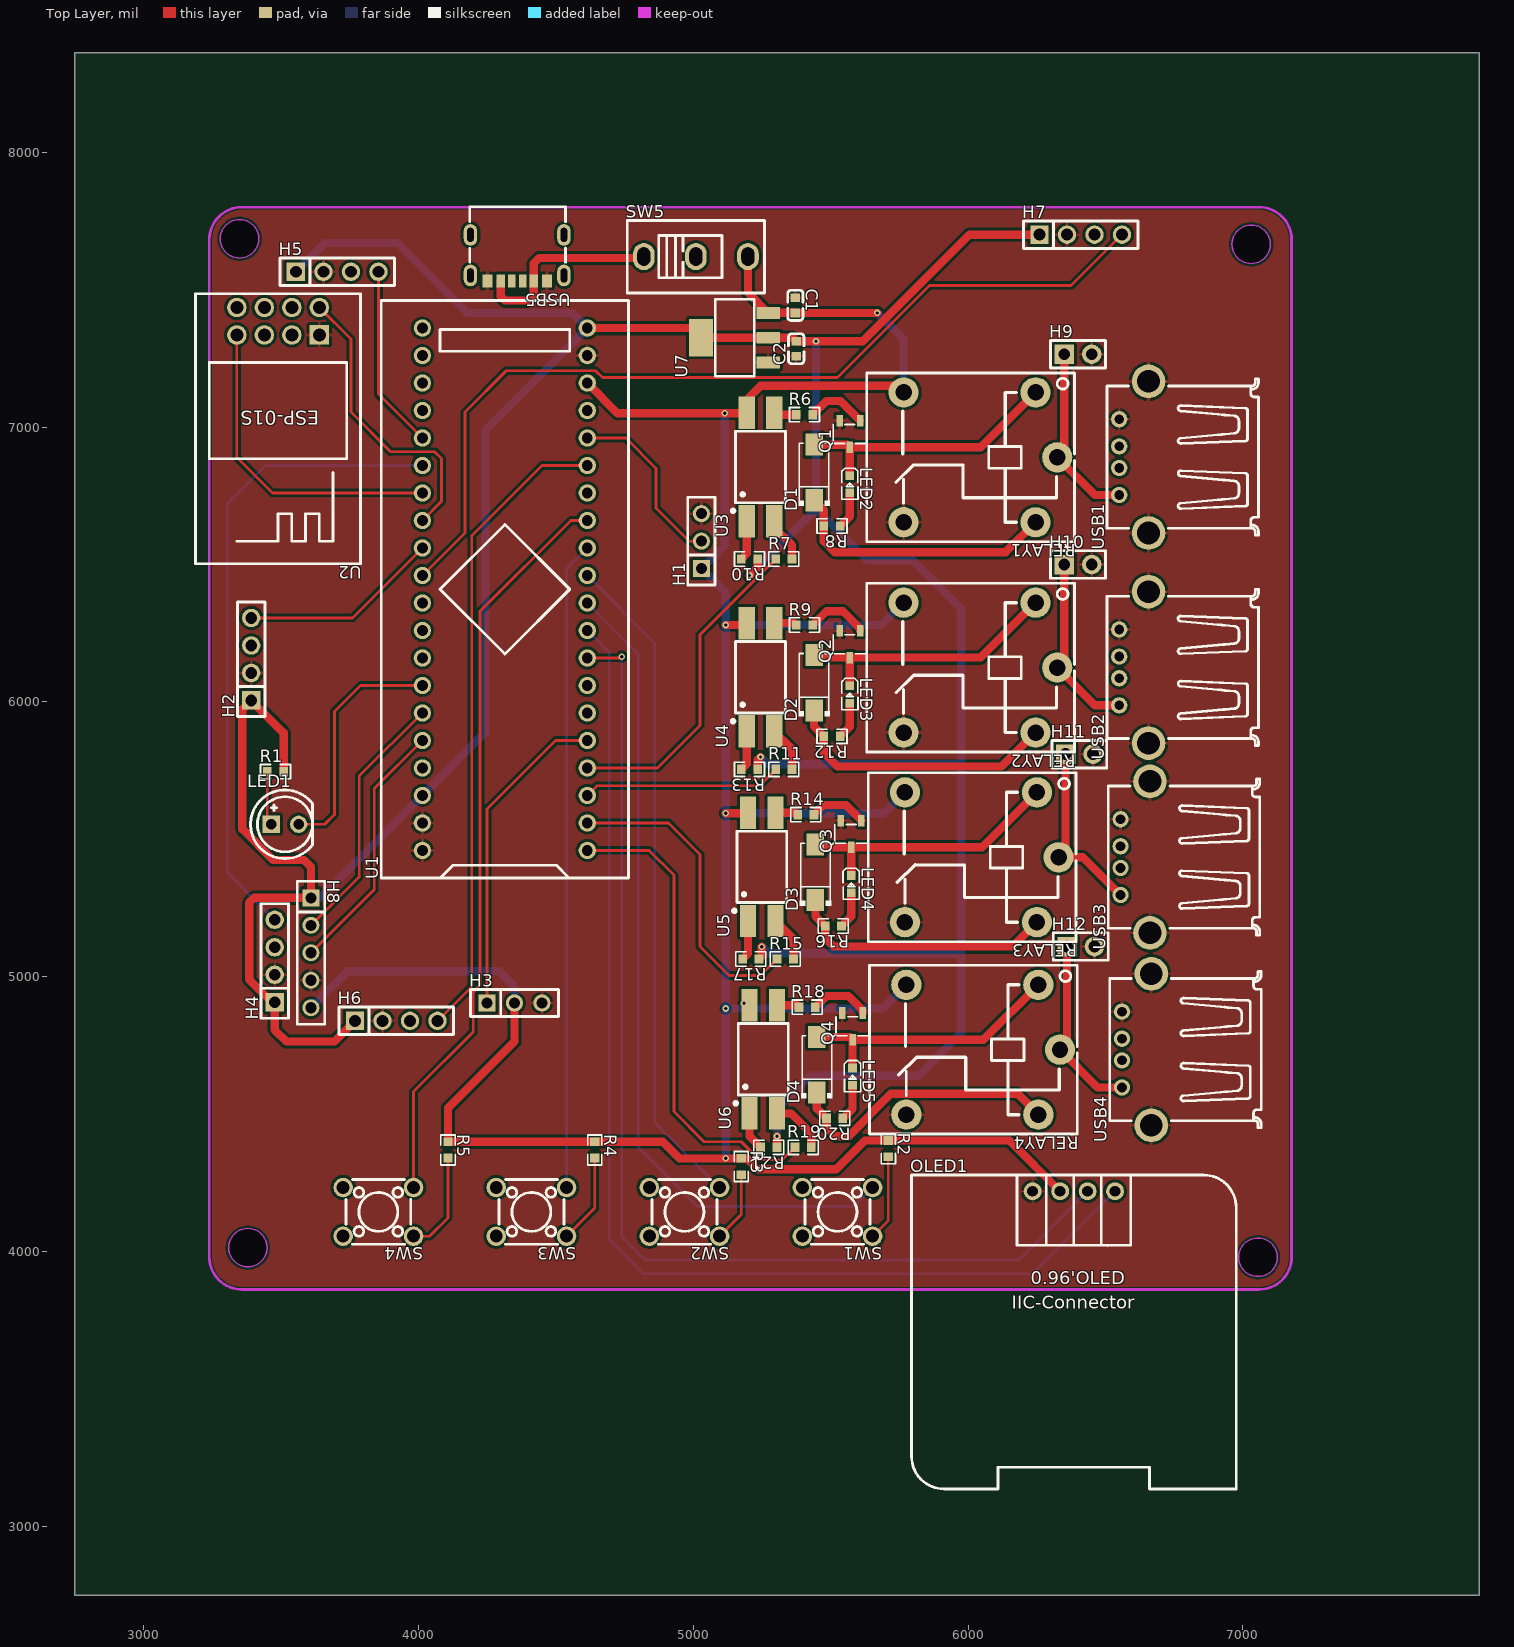
[diagram p0: Top Layer view]
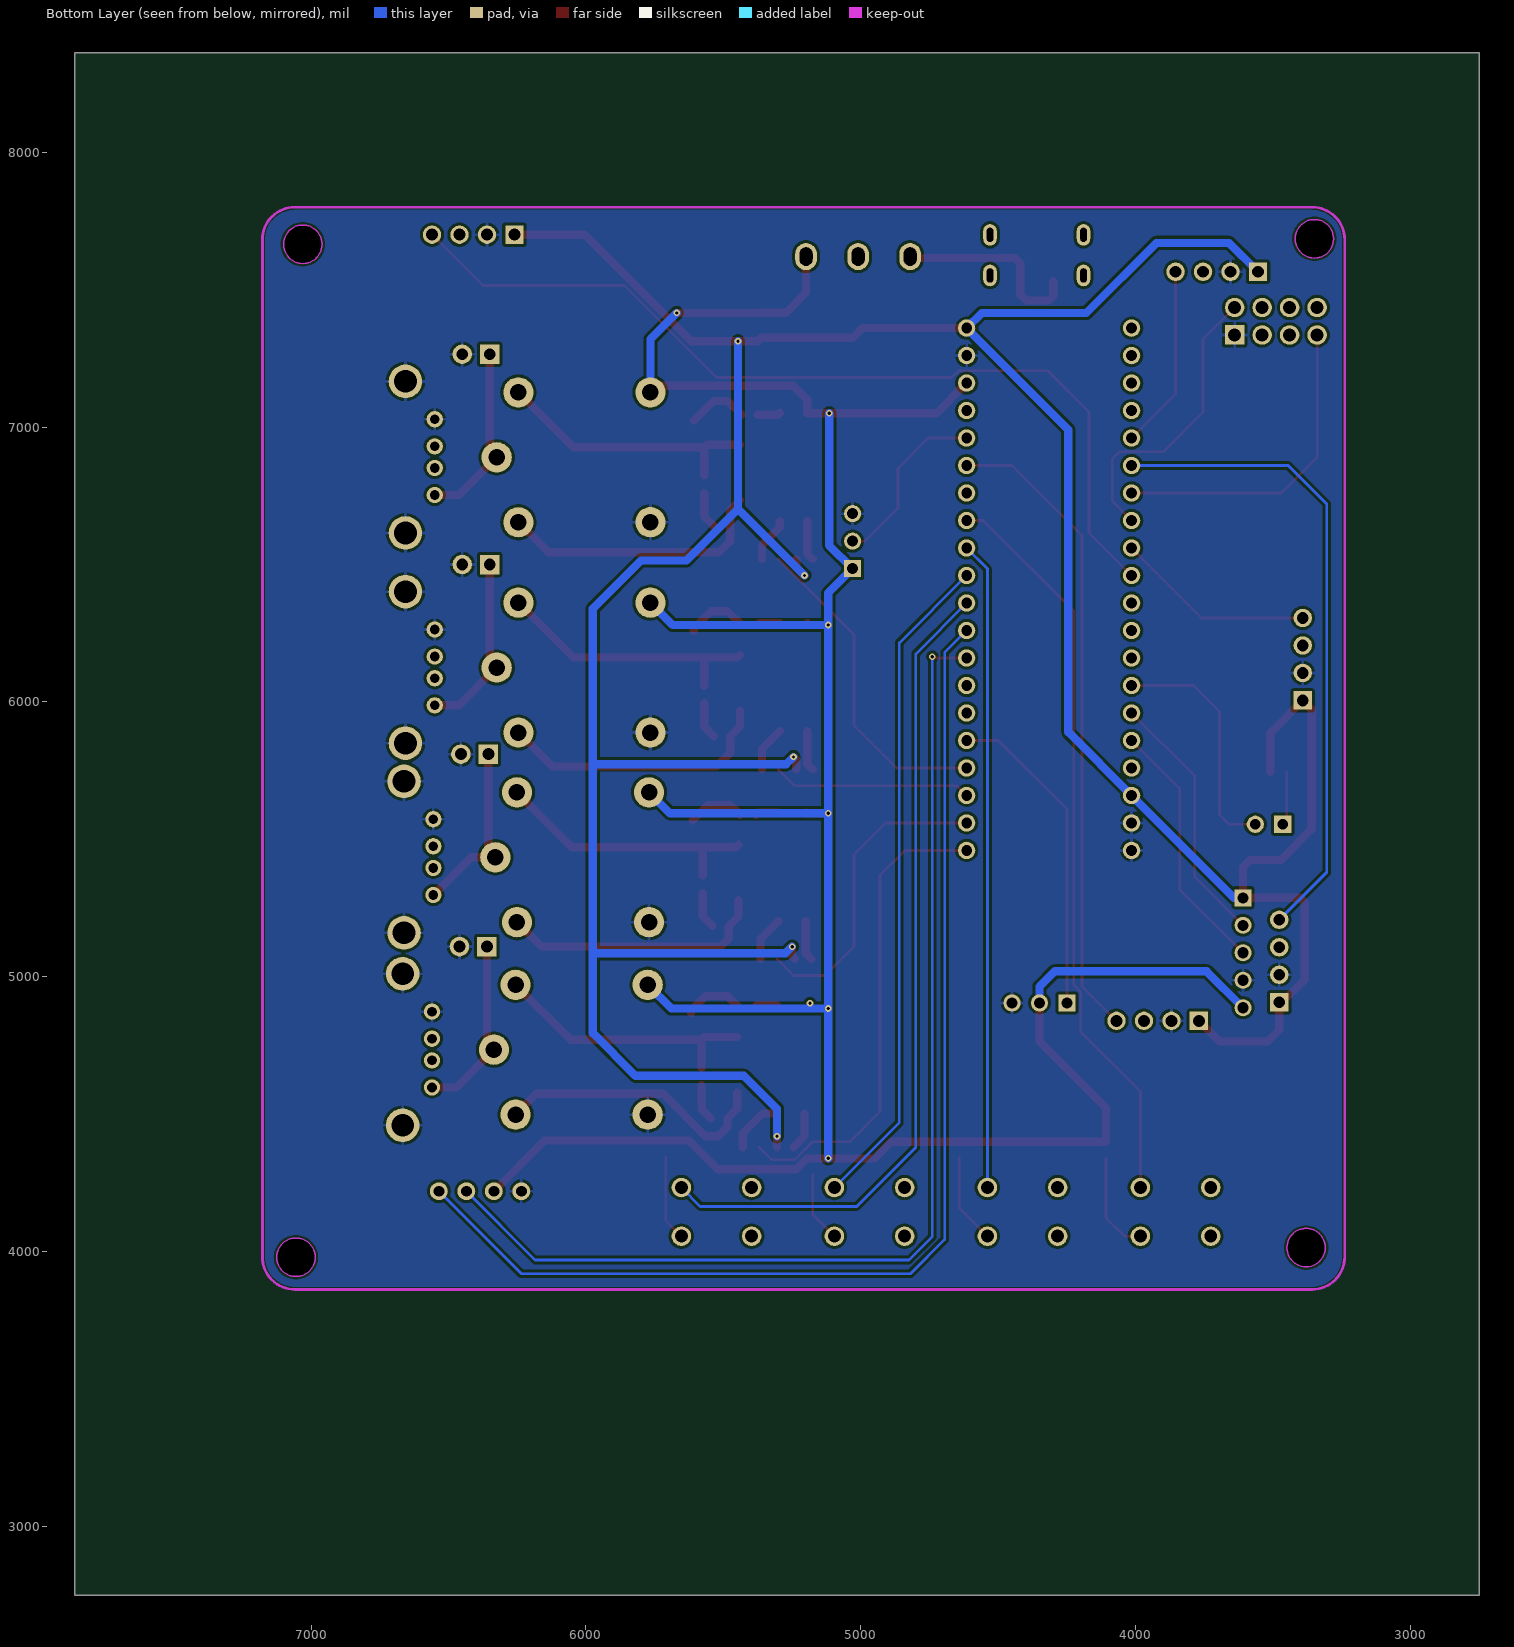
[diagram p1: Bottom Layer view, seen from below]
# Altium PCB MISC51241.pcbdoc
Units mil, origin at the board's own origin, x right, y up, seen from the top; angles counter-clockwise.
Board outline 5110 x 5612.11 mil, 2 copper layers (Top Layer, Bottom Layer), stack 62.206 mil thick; 70 components, 76 nets, 260 pads, 13 vias.

## Layer stack, top to bottom
Top Solder Mask Layer: solder mask 0.394, Dk 3.3
Top Layer: signal copper 1.379
Dielectric1: surface 59.449, FR4, Dk 4.5
Bottom Layer: signal copper 1.378
Bottom Solder Mask Layer: solder mask 0.394, Dk 3.3

## Board outline
7860,2750 2750,2750 2750,8362.11 7860,8362.11
cut-out: 3420,7685 cw(c3350,7685) 3280,7685 cw(c3350,7685)
cut-out: 3450,4015 cw(c3380,4015) 3310,4015 cw(c3380,4015)
cut-out: 7125,3980 cw(c7055,3980) 6985,3980 cw(c7055,3980)
cut-out: 7100,7665 cw(c7030,7665) 6960,7665 cw(c7030,7665)

## Design rules (kind name [scope] priority, off if disabled: settings)
BoardOutlineClearance copperThickness2oz_1 [All] p2 off: genericclearance=7.99 ignorepadtopadclearanceinfootprint=FALSE except(0: Arc-SplitContinuation Track-SplitContinuation SMDPad-SplitContinuation THPad-SplitContinuation Via-SplitContinuation Fill-SplitContinuation Region-SplitContinuation Poly-SplitContinuation Text-SplitContinuation Hole-SplitContinuation; 5.98: Arc-CutoutEdge Track-CutoutEdge SMDPad-CutoutEdge THPad-CutoutEdge Via-CutoutEdge Text-CutoutEdge; 6.9: Hole-OutlineEdge Hole-CutoutEdge; 10: Poly-OutlineEdge Poly-CutoutEdge; 11.81: Arc-OutlineEdge Track-OutlineEdge SMDPad-OutlineEdge THPad-OutlineEdge Via-OutlineEdge Fill-OutlineEdge Region-OutlineEdge Text-OutlineEdge Fill-CutoutEdge Region-CutoutEdge)
BoardOutlineClearance Plane_innerPlane_1 [All] p4 off: genericclearance=4.02 ignorepadtopadclearanceinfootprint=FALSE except(0: Arc-SplitContinuation Track-SplitContinuation SMDPad-SplitContinuation THPad-SplitContinuation Via-SplitContinuation Fill-SplitContinuation Region-SplitContinuation Poly-SplitContinuation Text-SplitContinuation Hole-SplitContinuation; 5.98: Arc-CutoutEdge Track-CutoutEdge SMDPad-CutoutEdge THPad-CutoutEdge Via-CutoutEdge Text-CutoutEdge; 6.9: Hole-OutlineEdge Hole-CutoutEdge; 10: Poly-OutlineEdge Poly-CutoutEdge; 11.81: Arc-OutlineEdge Track-OutlineEdge SMDPad-OutlineEdge THPad-OutlineEdge Via-OutlineEdge Fill-OutlineEdge Region-OutlineEdge Text-OutlineEdge Fill-CutoutEdge Region-CutoutEdge)
BoardOutlineClearance Copper_copperRegion_1 [All] p6 off: genericclearance=4.02 ignorepadtopadclearanceinfootprint=FALSE except(0: Arc-SplitContinuation Track-SplitContinuation SMDPad-SplitContinuation THPad-SplitContinuation Via-SplitContinuation Fill-SplitContinuation Region-SplitContinuation Poly-SplitContinuation Text-SplitContinuation Hole-SplitContinuation; 5.98: Arc-CutoutEdge Track-CutoutEdge SMDPad-CutoutEdge THPad-CutoutEdge Via-CutoutEdge Text-CutoutEdge; 6.9: Hole-OutlineEdge Hole-CutoutEdge; 10: Poly-OutlineEdge Poly-CutoutEdge; 11.81: Arc-OutlineEdge Track-OutlineEdge SMDPad-OutlineEdge THPad-OutlineEdge Via-OutlineEdge Fill-OutlineEdge Region-OutlineEdge Text-OutlineEdge Fill-CutoutEdge Region-CutoutEdge)
BoardOutlineClearance copperThickness1oz_1 [All] p8: genericclearance=4.02 ignorepadtopadclearanceinfootprint=FALSE except(0: Arc-SplitContinuation Track-SplitContinuation SMDPad-SplitContinuation THPad-SplitContinuation Via-SplitContinuation Fill-SplitContinuation Region-SplitContinuation Poly-SplitContinuation Text-SplitContinuation Hole-SplitContinuation; 5.98: Arc-CutoutEdge Track-CutoutEdge SMDPad-CutoutEdge THPad-CutoutEdge Via-CutoutEdge Text-CutoutEdge; 6.9: Hole-OutlineEdge Hole-CutoutEdge; 10: Poly-OutlineEdge Poly-CutoutEdge; 11.81: Arc-OutlineEdge Track-OutlineEdge SMDPad-OutlineEdge THPad-OutlineEdge Via-OutlineEdge Fill-OutlineEdge Region-OutlineEdge Text-OutlineEdge Fill-CutoutEdge Region-CutoutEdge)
Clearance copperThickness2oz [All] p1 off: gap=7.99 ignorepadtopadclearanceinfootprint=FALSE except(5.98: SMDPad-Track SMDPad-SMDPad THPad-Track SMDPad-THPad THPad-THPad Track-Via SMDPad-Via THPad-Via Via-Via Fill-SMDPad Region-SMDPad Fill-THPad Region-THPad Fill-Via Region-Via Fill-Fill Fill-Region Region-Region Arc-Track Arc-SMDPad Arc-THPad Arc-Via Fill-Arc Region-Arc Arc-Arc Text-Track SMDPad-Text Text-THPad Text-Via Fill-Text Region-Text Arc-Text Text-Text; 6.9: Hole-Track Hole-SMDPad Hole-THPad Hole-Via Fill-Hole Region-Hole Hole-Arc Hole-Text; 10: Poly-Track Poly-SMDPad Poly-THPad Poly-Via Poly-Fill Poly-Region Poly-Poly Poly-Arc Poly-Text Poly-Hole; 11.81: Fill-Track Region-Track)
Clearance Plane_innerPlane [All] p3 off: gap=4.02 ignorepadtopadclearanceinfootprint=FALSE except(5.98: SMDPad-Track SMDPad-SMDPad THPad-Track SMDPad-THPad THPad-THPad Track-Via SMDPad-Via THPad-Via Via-Via Fill-SMDPad Region-SMDPad Fill-THPad Region-THPad Fill-Via Region-Via Fill-Fill Fill-Region Region-Region Arc-Track Arc-SMDPad Arc-THPad Arc-Via Fill-Arc Region-Arc Arc-Arc Text-Track SMDPad-Text Text-THPad Text-Via Fill-Text Region-Text Arc-Text Text-Text; 6.9: Hole-Track Hole-SMDPad Hole-THPad Hole-Via Fill-Hole Region-Hole Hole-Arc Hole-Text; 10: Poly-Track Poly-SMDPad Poly-THPad Poly-Via Poly-Fill Poly-Region Poly-Poly Poly-Arc Poly-Text Poly-Hole; 11.81: Fill-Track Region-Track)
Clearance Copper_copperRegion [All] p5 off: gap=4.02 ignorepadtopadclearanceinfootprint=FALSE except(5.98: SMDPad-Track SMDPad-SMDPad THPad-Track SMDPad-THPad THPad-THPad Track-Via SMDPad-Via THPad-Via Via-Via Fill-SMDPad Region-SMDPad Fill-THPad Region-THPad Fill-Via Region-Via Fill-Fill Fill-Region Region-Region Arc-Track Arc-SMDPad Arc-THPad Arc-Via Fill-Arc Region-Arc Arc-Arc Text-Track SMDPad-Text Text-THPad Text-Via Fill-Text Region-Text Arc-Text Text-Text; 6.9: Hole-Track Hole-SMDPad Hole-THPad Hole-Via Fill-Hole Region-Hole Hole-Arc Hole-Text; 10: Poly-Track Poly-SMDPad Poly-THPad Poly-Via Poly-Fill Poly-Region Poly-Poly Poly-Arc Poly-Text Poly-Hole; 11.81: Fill-Track Region-Track)
Clearance copperThickness1oz [All] p7: gap=4.02 ignorepadtopadclearanceinfootprint=FALSE except(5.98: SMDPad-Track SMDPad-SMDPad THPad-Track SMDPad-THPad THPad-THPad Track-Via SMDPad-Via THPad-Via Via-Via Fill-SMDPad Region-SMDPad Fill-THPad Region-THPad Fill-Via Region-Via Fill-Fill Fill-Region Region-Region Arc-Track Arc-SMDPad Arc-THPad Arc-Via Fill-Arc Region-Arc Arc-Arc Text-Track SMDPad-Text Text-THPad Text-Via Fill-Text Region-Text Arc-Text Text-Text; 6.9: Hole-Track Hole-SMDPad Hole-THPad Hole-Via Fill-Hole Region-Hole Hole-Arc Hole-Text; 10: Poly-Track Poly-SMDPad Poly-THPad Poly-Via Poly-Fill Poly-Region Poly-Poly Poly-Arc Poly-Text Poly-Hole; 11.81: Fill-Track Region-Track)
DiffPairsRouting differentialPair [All] p1: maxlimit=6 minlimit=6 mostfreqgap=6 toplayer_minwidth=5 toplayer_prefwidth=10 toplayer_maxwidth=100 toplayer_mingap=6 toplayer_prefgap=6 toplayer_maxgap=6 bottomlayer_minwidth=5 bottomlayer_prefwidth=10 bottomlayer_maxwidth=100 bottomlayer_mingap=6 bottomlayer_prefgap=6 bottomlayer_maxgap=6 maxuncoupledlength=10
HoleToHoleClearance otherClearance [All] p1: gap=11.81 allowstackedmicrovias=TRUE
Length netLength [All] p1: minlimit=0 maxlimit=0
PasteMaskExpansion pasteMaskExpansion [All] p1: expansion=0
PlaneConnect innerPlane [All] p1: planeconnectstyle=Relief reliefexpansion=20 reliefentries=4 reliefconductorwidth=10 reliefairgap=10
PolygonConnect copperRegion [(InNet('GND'))] p1: connectstyle=Relief reliefconductorwidth=10 reliefentries=4 polygonreliefangle="90 Angle" airgapwidth=10 via.connectstyle=Relief via.reliefconductorwidth=10 via.reliefentries=4 via.polygonreliefangle="90 Angle" via.airgapwidth=10
RoutingVias viaSize [All] p1: holewidth=12.01 width=24.02 viastyle="Through Hole" minholewidth=11.81 minwidth=19.68 maxholewidth=248.03 maxwidth=393.7
SolderMaskExpansion solderMaskExpansion [IsVia] p1: expansion=-1000 istentingtop=TRUE
SolderMaskExpansion solderMaskExpansion [All] p2: expansion=2 istentingtop=FALSE
Width copperThickness2oz_2 [All] p1 off: maxlimit=100 minlimit=8 preferedwidth=10
Width copperThickness1oz_2 [All] p2: maxlimit=100 minlimit=5 preferedwidth=10

## Components (designator, comment, footprint, x,y, rotation, side; value= is the part's Value field where it differs from the comment)
C1 "100nF" C0603 5371.8,7442.75 r270 top
C2 "100nF" C0603 5375,7285 r90 top
D1 "US1M" SMA_L4.4-W2.8-LS5.4-RD 5440,6835 r90 top
D2 "US1M" SMA_L4.4-W2.8-LS5.4-RD 5440,6070 r90 top
D3 "US1M" SMA_L4.4-W2.8-LS5.4-RD 5445,5380 r90 top
D4 "US1M" SMA_L4.4-W2.8-LS5.4-RD 5450,4680 r90 top
H1 "" HDR-TH_3P-P2.54-V-F 5030,6585 r90 top
H2 "" HDR-TH_4P-P2.54-V-F 3392.37,6155.56 r90 top
H3 "" HDR-TH_3P-P2.54-V-F 4350,4905 r0 top
H4 "" HDR-TH_4P-P2.54-V-F 3477.85,5057.65 r90 top
H5 "" HDR-TH_4P-P2.54-V-F 3705,7565 r0 top
H6 "" HDR-TH_4P-P2.54-V-F 3920,4840 r0 top
H7 "" HDR-TH_4P-P2.54-V-F 6410,7700 r0 top
H8 "" HDR-TH_5P-P2.54-V-F 3609.58,5087.62 r270 top
H9 "" HDR-TH_2P-P2.54-V-M-1 6400,7265 r0 top
H10 "" HDR-TH_2P-P2.54-V-M-1 6400,6500 r0 top
H11 "" HDR-TH_2P-P2.54-V-M-1 6405,5810 r0 top
H12 "" HDR-TH_2P-P2.54-V-M-1 6410,5110 r0 top
LED1 "" LED-TH_5mm 3515,5555 r0 top
LED2 "" LED_0603 5570,6790 r270 top
LED3 "" LED_0603 5570,6025 r270 top
LED4 "" LED_0603 5575,5335 r270 top
LED5 "" LED_0603 5580,4635 r270 top
OLED1 "" 0.96OLED_4P 6385,4220 r0 top
Q1 "S8050" SOT-23-3_L2.9-W1.6-P1.90-LS2.8-BR 5570,6975 r90 top
Q2 "S8050" SOT-23-3_L2.9-W1.6-P1.90-LS2.8-BR 5570,6210 r90 top
Q3 "S8050" SOT-23-3_L2.9-W1.6-P1.90-LS2.8-BR 5575,5520 r90 top
Q4 "S8050" SOT-23-3_L2.9-W1.6-P1.90-LS2.8-BR 5580,4820 r90 top
R1 "10K" R0603 3480.68,5746.32 r0 top
R2 "10K" R0603 5710,4375 r270 top
R3 "10K" R0603 5175,4310 r270 top
R4 "10K" R0603 4641.97,4370.3 r270 top
R5 "10K" R0603 4107.95,4370.3 r270 top
R6 "1kΩ" R0603 5405,7045 r0 top
R7 "470Ω" R0603 5330,6520 r0 top
R8 "4.7kΩ" R0603 5505,6640 r180 top
R9 "1kΩ" R0603 5405,6280 r0 top
R10 "1kΩ" R0603 5205,6520 r180 top
R11 "470Ω" R0603 5330,5755 r0 top
R12 "4.7kΩ" R0603 5505,5875 r180 top
R13 "1kΩ" R0603 5205,5755 r180 top
R14 "1kΩ" R0603 5410,5590 r0 top
R15 "470Ω" R0603 5335,5065 r0 top
R16 "4.7kΩ" R0603 5510,5185 r180 top
R17 "1kΩ" R0603 5210,5065 r180 top
R18 "1kΩ" R0603 5415,4890 r0 top
R19 "470Ω" R0603 5400,4380 r0 top
R20 "4.7kΩ" R0603 5515,4485 r180 top
R21 "1kΩ" R0603 5275,4380 r180 top
RELAY1 "SRD-12VDC-SL-C" RELAY-TH_SRD-XXVDC-XL-C 6045,6890 r180 top
RELAY2 "SRD-12VDC-SL-C" RELAY-TH_SRD-XXVDC-XL-C 6045,6125 r180 top
RELAY3 "SRD-12VDC-SL-C" RELAY-TH_SRD-XXVDC-XL-C 6050,5435 r180 top
RELAY4 "SRD-12VDC-SL-C" RELAY-TH_SRD-XXVDC-XL-C 6055,4735 r180 top
SW1 "" SW-TH_4P-L6.0-W6.0-P4.50-LS6.5 5525,4145 r180 top
SW2 "" SW-TH_4P-L6.0-W6.0-P4.50-LS6.5 4968.33,4145 r180 top
SW3 "" SW-TH_4P-L6.0-W6.0-P4.50-LS6.5 4411.67,4145 r180 top
SW4 "" SW-TH_4P-L6.0-W6.0-P4.50-LS6.5 3855,4145 r180 top
SW5 "XY-SS12D10L3" SW-TH_3P-L12.7-W6.7_XY-SS12D10LXX 5010,7620 r0 top
U1 "STM32F103C8T6-Card" CONN-TH_L53.3-W22.9_STM32F103C8T6-CARD 4315,6410 r90 top
U2 "ESP-01S" WIFIM-TH_ESP-01S 3490,7385 r180 top
U3 "PC817C" OPTO-SMD-4_L4.6-W6.5-P2.54-LS10.3-TL 5245,6855 r90 top
U4 "PC817C" OPTO-SMD-4_L4.6-W6.5-P2.54-LS10.3-TL 5245,6090 r90 top
U5 "PC817C" OPTO-SMD-4_L4.6-W6.5-P2.54-LS10.3-TL 5250,5400 r90 top
U6 "PC817C" OPTO-SMD-4_L4.6-W6.5-P2.54-LS10.3-TL 5255,4700 r90 top
U7 "" SOT_223 5150,7325 r90 top
USB1 "" "USB_ Type-A" 6765,6890 r90 top
USB2 "" "USB_ Type-A" 6765,6125 r90 top
USB3 "" "USB_ Type-A" 6770,5435 r90 top
USB4 "" "USB_ Type-A" 6775,4735 r90 top
USB5 "" "USB_ TYPE-C-6P" 4365,7615 r180 top

## Footprints (in the part's own frame and the unit in brackets; to place one, negate y for a bottom-side part, rotate by r counter-clockwise, add the part's x,y. Pads: shape width x height; smd on the part's side, far side on the other; paste and mask are expansions set on the pad)
0.96OLED_4P [mm]
  round 1.65 hole 1 copper offset 0,0: 1(-3.81,-0.001) 2(-1.27,0.002) 3(1.27,0.002) 4(3.81,0.002)
  silkscreen extent -15,-27.5 15,1.5
C0603 [mm]
  rect 0.8x0.9 smd: 1(-0.7,0) 2(0.7,0)
  silkscreen extent -1.39,-0.71 1.39,0.71
CONN-TH_L53.3-W22.9_STM32F103C8T6-CARD [mm]
  round 1.6 hole 1: 1(-24.13,-7.62) 2(-21.59,-7.62) 3(-19.05,-7.62) 4(-16.51,-7.62) 5(-13.97,-7.62) 6(-11.43,-7.62) 7(-8.89,-7.62) 8(-6.35,-7.62) 9(-3.81,-7.62) 10(-1.27,-7.62) 11(1.27,-7.62) 12(3.81,-7.62) 13(6.35,-7.62) 14(8.89,-7.62) 15(11.43,-7.62) 16(13.97,-7.62) 17(16.51,-7.62) 18(19.05,-7.62) 19(21.59,-7.62) 20(24.13,-7.62) 21(24.13,7.62) 22(21.59,7.62) 23(19.05,7.62) 24(16.51,7.62) 25(13.97,7.62) 26(11.43,7.62) 27(8.89,7.62) 28(6.35,7.62) 29(3.81,7.62) 30(1.27,7.62) 31(-1.27,7.62) 32(-3.81,7.62) 33(-6.35,7.62) 34(-8.89,7.62) 35(-11.43,7.62) 36(-13.97,7.62) 37(-16.51,7.62) 38(-19.05,7.62) 39(-21.59,7.62) 40(-24.13,7.62)
  silkscreen extent -26.67,-11.43 26.67,11.43
HDR-TH_2P-P2.54-V-M-1 [mm]
  rect 1.8x1.8 hole 1.1: 1(-1.27,0)
  round 1.8 hole 1.1: 2(1.27,0)
  silkscreen extent -2.54,-1.27 2.54,1.27
HDR-TH_3P-P2.54-V-F [mil]
  rect 62x62 hole 40.16: 1(-100,0)
  round 62 hole 40.16: 2(0,0) 3(100,0)
  silkscreen extent -160,-49 160,49
HDR-TH_4P-P2.54-V-F [mm]
  rect 1.7x1.7 hole 1.1: 1(-3.81,0)
  round 1.7 hole 1.1: 2(-1.27,0) 3(1.27,0) 4(3.81,0)
  silkscreen extent -5.29,-1.27 5.29,1.27
HDR-TH_5P-P2.54-V-F [mil]
  rect 62x62 hole 40.16: 1(-200,0)
  round 62 hole 40.16: 2(-100,0) 3(0,0) 4(100,0) 5(200,0)
  silkscreen extent -260,-50 260,50
LED-TH_5mm [mm]
  rect 1.6x1.6 hole 1 paste+0 mask+0.051: 1(-1.27,0)
  round 1.6 hole 1 paste+0 mask+0.051: 2(1.27,0)
  silkscreen extent -3.17,-3.17 2.54,3.17
LED_0603 [mil]
  rect 31.5x31.5 smd paste+0 mask+2: 1(-33.5,-0.4) 2(29.5,-0.2)
  silkscreen extent -61,-30 53,30
OPTO-SMD-4_L4.6-W6.5-P2.54-LS10.3-TL [mm]
  rect 3x1.5 smd: 1(-5,1.27) 2(-5,-1.27) 3(5,-1.27) 4(5,1.27)
  silkscreen extent -4.21,-2.3 3.3,2.69
R0603 [mil]
  rect 31.75x34.02 smd paste-3937.01 mask+2: 1(-29.66,0) 2(29.66,0)
  silkscreen extent -55,-26 55,26
RELAY-TH_SRD-XXVDC-XL-C [mil]
  round 110 hole 60: 1(-200.79,-236.22) 2(279.53,-236.2) 3(279.53,236.2) 4(-200.79,236.22) 5(-279.53,0)
  silkscreen extent -342,-307 413,307
SMA_L4.4-W2.8-LS5.4-RD [mil]
  rect 80.57x63.78 smd: 1(-101,0) 2(101,0)
  silkscreen extent -121,-57 106,57
SOT-23-3_L2.9-W1.6-P1.90-LS2.8-BR [mm]
  rect 1.07x0.6 smd: 1(1.235,-0.95) 2(1.235,0.95) 3(-1.235,0)
  silkscreen extent -0.88,-1.54 0.88,1.54
SOT_223 [mil]
  rect 43.3x86.6 smd paste+0 mask+2: 1(-90.5,-123.05) 2(0,-123.05) 3(90.6,-123.05)
  rect 137.8x86.6 smd paste+0 mask+2: 4(0,120.95)
  silkscreen extent -140,-72 140,70
SW-TH_3P-L12.7-W6.7_XY-SS12D10LXX [mm]
  oval 2x2.5 hole 1.2 slot 1.7 at 90 deg: 1(-4.81,0) 2(0,0) 3(4.81,0)
  silkscreen extent -6.35,-3.35 6.35,3.35
SW-TH_4P-L6.0-W6.0-P4.50-LS6.5 [mm]
  round 1.8 hole 1.2: 1(-3.25,2.25) 2(3.25,2.25) 3(-3.25,-2.25) 4(3.25,-2.25)
  silkscreen extent -3,-3 3,3
"USB_ Type-A" [mm]
  round 1.5 hole 0.9 copper offset 0,0 paste+0 mask+0.051: 1(-3.484,5.461) 4(3.516,5.461)
  round 1.5 hole 0.9 paste+0 mask+0.051: 2(-0.984,5.461) 3(1.016,5.461)
  round 3.1 hole 2.1 paste+0 mask+0.051: SH1(7.016,2.751) SH2(-6.984,2.751)
  silkscreen extent -7.2,-7.4 7.24,6.6
"USB_ TYPE-C-6P" [mm]
  oval 1.25x2 hole 0.6 slot 1.3 at 90 deg paste+0 mask+0.05: 7(-4.193,1.611) 8(4.447,1.611) 9(-4.193,-2.139) 10(4.447,-2.139)
  rect 0.7x1.2 smd paste-100 mask+0.05: A5(-0.373,2.139) B5(0.627,2.139)
  rect 0.8x1.2 smd paste-100 mask+0.05: A9(1.647,2.139) B9(-1.393,2.139)
  rect 0.9x1.2 smd paste-100 mask+0.05: A12(2.877,2.139) B12(-2.623,2.139)
  silkscreen extent -4.34,-4.75 4.52,0.39
WIFIM-TH_ESP-01S [mm]
  rect 1.8x1.8 hole 1.2: 1(-3.81,1.27)
  round 1.8 hole 1.2: 2(-1.27,1.27) 3(1.27,1.27) 4(3.81,1.27) 5(3.81,-1.27) 6(1.27,-1.27) 7(-1.27,-1.27) 8(-3.81,-1.27)
  silkscreen extent -7.62,-2.54 7.62,22.4

## Via types
v1: diameter 24.02, hole 12, Top Layer to Bottom Layer, 13 vias

## Nets (pads, with @x,y where several pads share a name; then routed paths per layer and width w, separated by ;. In a path a pad name is that pad's centre, name@x,y a point inside that pad or via, vN(x,y) a via of type N, cw(c..) or ccw(c..) an arc to the next point about the centre after c; other vN are vias at no path point)
3V3: U2.5
$1N17156: LED1.1 R1.1 | length 197.1
  Top Layer w10: R1.1 3451.02,5568.98 LED1.1
$1N17164: R2.2 SW1.1 | length 312.6
  Top Layer w10: SW1.1 5710,4113.47 R2.2
$1N17166: R3.2 SW2.1 | length 256.5
  Top Layer w10: SW2.1 5175,4135.14 R3.2
$1N17168: R4.2 SW3.1 | length 326.6
  Top Layer w10: SW3.1 4641.97,4158.77 R4.2
$1N17170: R5.2 SW4.1 | length 370.2
  Top Layer w10: SW4.1 4041.42,4056.42 4107.95,4122.95 R5.2
$1N17175: R10.2 U3.1 | length 146.3
  Top Layer w30: R10.2 5195,6539.66 U3.1
$1N17179: R6.1 U3.3 | length 83.2
  Top Layer w30: U3.3 5301.85,7045 R6.1
$1N17180: Q1.1 R6.2 | length 223
  Top Layer w30: R6.2 5484.66,7095 5536.02,7095 Q1.1
$1N17182: D1.2 LED2.1 Q1.3 RELAY1.1 | length 995.6
  Top Layer w30: D1.2 5560.38,6936 Q1.3 ; LED2.1 5570,6823.9 Q1.3 ; RELAY1.1 6045.94,6926.38 Q1.3
$1N17183: D1.1 R8.2 RELAY1.4 | length 995.9
  Top Layer w30: D1.1 5475.34,6698.66 R8.2 5475.34,6584.66 5515,6545 6137.01,6545 RELAY1.4
$1N17187: R7.2 U3.2 | length 164.9
  Top Layer w30: U3.2 5295,6635 5359.66,6570.34 R7.2
$1N17191: H9.1 RELAY1.5 USB1.1 | length 667.8
  Top Layer w30: H9.1 6350,6915.47 RELAY1.5 6461.7,6752.83 USB1.1
$1N17198: H10.1 RELAY2.5 USB2.1 | length 667.8
  Top Layer w30: H10.1 6350,6150.47 RELAY2.5 6461.7,5987.83 USB2.1
$1N17201: R11.2 U4.2 | length 164.9
  Top Layer w30: U4.2 5359.66,5828.49 R11.2
$1N17203: R13.2 U4.1 | length 146.3
  Top Layer w30: R13.2 5195,5774.66 U4.1
$1N17206: R9.1 U4.3 | length 83.2
  Top Layer w30: U4.3 5368.49,6286.85 R9.1
$1N17207: Q2.1 R9.2 | length 228.3
  Top Layer w30: R9.2 5484.66,6330 5545,6330 5607.4,6267.6 Q2.1
$1N17209: D2.2 LED3.1 Q2.3 RELAY2.1 | length 995.6
  Top Layer w30: D2.2 5449.62,6161.38 Q2.3 ; LED3.1 5570,6058.9 Q2.3 ; RELAY2.1 6045.94,6161.38 Q2.3
$1N17210: D2.1 R12.2 RELAY2.4 | length 1011.3
  Top Layer w30: D2.1 5440,5910.34 R12.2 5475.34,5814.66 5525,5765 6122.01,5765 RELAY2.4
$1N17214: H11.1 RELAY3.5 USB3.1 | length 667.8
  Top Layer w30: H11.1 6355,5460.47 RELAY3.5 6417.83,5435 USB3.1
$1N17217: R15.2 U5.2 | length 164.9
  Top Layer w30: U5.2 5364.66,5138.49 R15.2
$1N17219: R17.2 U5.1 | length 146.3
  Top Layer w30: R17.2 5200,5084.66 U5.1
$1N17222: R14.1 U5.3 | length 83.2
  Top Layer w30: U5.3 5373.49,5596.85 R14.1
$1N17223: Q3.1 R14.2 | length 210.6
  Top Layer w30: R14.2 5474.66,5625 5556.02,5625 Q3.1
$1N17225: D3.2 LED4.1 Q3.3 RELAY3.1 | length 995.6
  Top Layer w30: D3.2 5454.62,5471.38 Q3.3 ; LED4.1 5575,5368.9 Q3.3 ; RELAY3.1 6050.94,5471.38 Q3.3
$1N17226: D3.1 R16.2 RELAY3.4 | length 973.5
  Top Layer w30: D3.1 5445,5220.34 R16.2 5480.34,5139.66 5510,5110 6162.01,5110 RELAY3.4
$1N17230: H12.1 RELAY4.5 USB4.1 | length 667.8
  Top Layer w30: H12.1 6360,4760.47 RELAY4.5 6471.7,4597.83 USB4.1
$1N17233: R19.2 U6.2 | length 205.2
  Top Layer w30: U6.2 5356.85,4503.15 5429.66,4430.34 R19.2
$1N17235: R21.2 U6.1 | length 139.9
  Top Layer w30: U6.1 5205,4420.34 R21.2
$1N17238: R18.1 U6.3 | length 83.2
  Top Layer w30: U6.3 5378.49,4896.85 R18.1
$1N17239: Q4.1 R18.2 | length 220
  Top Layer w30: R18.2 5484.66,4930 5565,4930 5617.4,4877.6 Q4.1
$1N17241: D4.2 LED5.1 Q4.3 RELAY4.1 | length 995.6
  Top Layer w30: D4.2 5570.38,4781 Q4.3 ; LED5.1 5580,4668.9 Q4.3 ; RELAY4.1 6055.94,4771.38 Q4.3
$1N17242: D4.1 R20.2 RELAY4.4 | length 1019.6
  Top Layer w30: D4.1 5450,4520.34 R20.2 5485.34,4454.66 5520,4420 5565,4420 5720,4575 6179.57,4575 RELAY4.4
$1N17253: LED2.2 R8.1 | length 135.1
  Top Layer w30: R8.1 5569.8,6675.14 LED2.2
$1N17254: LED3.2 R12.1 | length 135.1
  Top Layer w30: R12.1 5569.8,5910.14 LED3.2
$1N17255: LED4.2 R16.1 | length 135.1
  Top Layer w30: R16.1 5574.8,5220.14 LED4.2
$1N17256: LED5.2 R20.1 | length 135.1
  Top Layer w30: R20.1 5579.8,4520.14 LED5.2
+5V: C1.2 H1.1 H3.2 H8.5 OLED1.2 R2.1 R3.1 R4.1 R5.1 RELAY1.2 RELAY2.2 RELAY3.2 RELAY4.2 SW5.3 U1.18 U3.4 U4.4 U5.4 U6.4 U7.3 | length 11106.6
  Top Layer w30: H3.2 4350,4765 4107.95,4522.95 R5.1 R4.1 4890.04,4399.96 4950.34,4339.66 v1(5118.88,4339.66) R3.1 5195.34,4339.66 5235,4300 5520,4300 5624.66,4404.66 R2.1 6150.39,4404.66 OLED1.2@6335,4220.05 ; U1.18 4725,7050 v1(5115,7050) 5193.15,7050 U3.4 5195,7100 5245,7150 5741.67,7150 RELAY1.2 ; v1(5118.88,5595) 5198.15,5595 U5.4 ; v1(5118.88,6280) 5188.15,6280 U4.4 ; SW5.3 5199.37,7489.28 U7.3 5371.39,7415.6 C1.2 v1(5670,7415.19)
  Bottom Layer w30: H8.5 3741.95,5020 4295,5020 4350,4965 H3.2 ; v1(5115,7050) 5115,6570 H1.1 5118.88,6396.12 v1(5118.88,6280) ; v1(5118.88,4339.66) v1(5118.88,4885) ; v1(5670,7415.19) 5765.47,7319.72 RELAY1.2 ; RELAY2.2 5684.27,6280 v1(5118.88,6280) ; RELAY3.2 5694.27,5595 v1(5118.88,5595) ; RELAY4.2 5689.27,4885 v1(5118.88,4885) ; v1(5118.88,4885) v1(5118.88,5595) ; v1(5118.88,5595) v1(5118.88,6280)
  other v1: 5185,4904.37
GND: C1.1 C2.1 H1.3 H2.2 H3.3 H4.2 H5.2 H6.2 H7.2 H8.4 H9.2 H10.2 H11.2 H12.2 OLED1.1 Q1.2 Q2.2 Q3.2 Q4.2 RELAY1.3 RELAY2.3 RELAY3.3 RELAY4.3 U1.19 U1.39 U1.40 U2.1 U7.1 USB1.4 USB1.SH1 USB1.SH2 USB2.4 USB2.SH1 USB2.SH2 USB3.4 USB3.SH1 USB3.SH2 USB4.4 USB4.SH1 USB4.SH2 USB5.A12 USB5.B12
IN: SW5.1 USB5.A9 USB5.B9 | length 715.1
  Top Layer w30: USB5.A9 4300.16,7474.84 4315,7460 4398.05,7460 4419.84,7481.79 USB5.B9 4419.84,7594.84 4440,7615 4815.63,7615 SW5.1
NRST: U1.37
PA0: H5.4 U1.25 | length 671.3
  Top Layer w10: H5.4 3855,7120 U1.25
PA1: H4.4 U1.26 | length 2351.9
  Bottom Layer w10: H4.4 3305,5380.5 3305,6720 3445,6860 U1.26
PA2: U1.27 U2.4 | length 1173.8
  Top Layer w10: U2.4 3340,6890 3470,6760 U1.27
PA3: U1.28 U2.8 | length 1082
  Top Layer w10: U2.8 3755,7320 3755,7055 3900,6910 4060,6910 4085,6885 4085,6730 U1.28
PA4: H2.4 U1.29 | length 728
  Top Layer w10: H2.4 3760.55,6305.56 U1.29
PA5: H7.4 U1.30 | length 3337.1
  Top Layer w10: U1.30 4170,6615 4170,7055 4320,7205 4645,7205 4670,7180 5525,7180 5860,7515 6375,7515 H7.4
PA6: U1.31
PA7: U1.32
PA8: H3.1 U1.5 | length 1173.6
  Top Layer w10: H3.1 4250,5610 4500,5860 U1.5
PA9: U1.6
PA10: U1.7
PA11: OLED1.3 U1.8 | length 4070.9
  Top Layer w10: U1.8 4735,6160 v1(4740,6165)
  Bottom Layer w10: v1(4740,6165) 4740,4055 4825,3970 6184.95,3970 OLED1.3@6435,4220.05
PA12: OLED1.4 U1.9 | length 4264.2
  Bottom Layer w10: U1.9 4695,6180 4695,4045 4820,3920 6234.95,3920 OLED1.4@6535,4220.05
PA15: SW1.3 U1.10 | length 3027
  Bottom Layer w10: U1.10 4800,6175 4800,4380 5015,4165 5584.37,4165 SW1.3
PB0: U1.33
PB1: LED1.2 U1.34 | length 878.8
  Top Layer w10: LED1.2 3660,5555 3695,5590 3695,5965 3790,6060 U1.34
PB3: SW2.3 U1.11 | length 2425.8
  Bottom Layer w10: U1.11 4860,6215 4860,4469.86 SW2.3
PB4: SW3.3 U1.12 | length 2357.6
  Bottom Layer w10: SW3.3 4539.62,6484.62 U1.12
PB5: SW4.3 U1.13 | length 2723.4
  Top Layer w10: SW4.3 3982.95,4582.95 4200,4800 4200,4945 4225,4970 4225,6330 4555,6660 U1.13
PB6: U1.14
PB7: H6.4 U1.15 | length 2342.4
  Top Layer w10: H6.4 4195,4965 4195,6605 4450,6860 U1.15
PB8: H1.2 U1.16 | length 655.3
  Top Layer w10: U1.16 4755,6960 4865,6850 4865,6705 4985,6585 H1.2
PB9: U1.17
PB10: H8.2 U1.35 | length 940.3
  Top Layer w10: H8.2 3785,5363.05 3785,5730 U1.35
PB11: H8.3 U1.36 | length 940.3
  Top Layer w10: H8.3 3840,5318.05 3840,5685 U1.36
PB12: R19.1 U1.1 | length 1743.7
  Top Layer w10: U1.1 4840,5460 4930,5370 4930,4510 5040,4400 5175,4400 5240,4335 5325.34,4335 R19.1
PB13: R15.1 U1.2 | length 1141.3
  Top Layer w10: U1.2 4910,5560 5025,5445 5025,5110 5130,5005 5245.34,5005 R15.1
PB14: R11.1 U1.3 | length 724.7
  Top Layer w10: U1.3 4650,5695 5240.34,5695 R11.1
PB15: R7.1 U1.4 | length 1193.3
  Top Layer w10: U1.4 4870,5760 5025,5915 5025,6244.66 R7.1
PC13: U1.22
PC14: U1.23
PC15: U1.24
VBAT: U1.21
VCC: C2.2 H2.1 H4.1 H5.1 H6.1 H7.1 H8.1 R1.2 R10.1 R13.1 R17.1 R21.1 U1.20 U1.38 U7.2 U7.4 | length 13600.7
  Top Layer w30: R1.2 3510.34,5887.59 H2.1 3360,5973.18 3360,5537.2 3471.67,5425.53 3584.47,5425.53 3609.58,5400.42 H8.1 3402.62,5287.62 3385,5270 3385,4990 3467.35,4907.65 H4.1 3477.85,4807.15 3520,4765 3695,4765 H6.1 ; U1.20 4994.05,7360 U7.4 U7.2 5362.56,7325 C2.2 v1(5446.89,7312.56) 5617.56,7312.56 6005,7700 H7.1 ; v1(5205,6460) 5234.66,6489.66 R10.1 ; R13.1 5234.66,5789.66 v1(5245,5800) ; R17.1 5250,5075.34 v1(5250,5110) ; R21.1 5305,4380.34 v1(5305,4420)
  Bottom Layer w30: H5.1 3660,7670 3925,7670 4180,7415 4560,7415 U1.20 4245,6990 4245,5890 U1.38 3642.62,5287.62 H8.1 ; v1(5205,6460) 5446.89,6701.89 ; v1(5245,5800) 5271.62,5773.38 5975,5773.38 ; v1(5250,5110) 5273.87,5086.13 5975,5086.13 ; v1(5305,4420) 5305,4520 5425,4640 5820,4640 5975,4795 5975,5086.13 ; v1(5446.89,7312.56) 5446.89,6701.89 ; 5446.89,6701.89 5633.77,6515 5800,6515 5975,6340 5975,5773.38 ; 5975,5086.13 5975,5773.38
pads on no net: H2.3 H4.3 H5.3 H6.3 H7.3 SW1.2 SW1.4 SW2.2 SW2.4 SW3.2 SW3.4 SW4.2 SW4.4 SW5.2 U2.2 U2.3 U2.6 U2.7 USB1.2 USB1.3 USB2.2 USB2.3 USB3.2 USB3.3 USB4.2 USB4.3 USB5.7 USB5.8 USB5.9 USB5.10 USB5.A5 USB5.B5

## Polygon pours and split planes (outlines as drawn)
GND on Top Layer (solid, remove dead copper, pour order 0): 3000,8045 3000,3595 7530,3595 7530,8045
GND on Bottom Layer (solid, remove dead copper, pour order 2): 3010,7985 3010,3650 7610,3650 7610,7985

## Keep-outs
Board Outline Layer:
  region: 3420,7685 cw(c3350,7685) 3280,7685 cw(c3350,7685)
  circle w0.1: c3350,7685 r70
  region: 3420,7685 3419.62,7677.68 3418.47,7670.45 3416.57,7663.37 3413.95,7656.53 3410.62,7650 3406.63,7643.85 3402.02,7638.16 3396.84,7632.98 3391.14,7628.37 3385,7624.38 3378.47,7621.05 3371.63,7618.43 3364.55,7616.53 3357.32,7615.38 3350,7615 3342.68,7615.38 3335.45,7616.53 3328.37,7618.43 3321.53,7621.05 3315,7624.38 3308.86,7628.37 3303.16,7632.98 3297.98,7638.16 3293.37,7643.85 3289.38,7650 3286.05,7656.53 3283.43,7663.37 3281.53,7670.45 3280.38,7677.68 3280,7685 3280.38,7692.32 3281.53,7699.55 3283.43,7706.63 3286.05,7713.47 3289.38,7720 3293.37,7726.15 3297.98,7731.84 3303.16,7737.02 3308.86,7741.63 3315,7745.62 3321.53,7748.95 3328.37,7751.57 3335.45,7753.47 3342.68,7754.62 3350,7755 3357.32,7754.62 3364.55,7753.47 3371.63,7751.57 3378.47,7748.95 3385,7745.62 3391.14,7741.63 3396.84,7737.02 3402.02,7731.84 3406.63,7726.15 3410.62,7720 3413.95,7713.47 3416.57,7706.63 3418.47,7699.55 3419.62,7692.32
  region: 3450,4015 cw(c3380,4015) 3310,4015 cw(c3380,4015)
  circle w0.1: c3380,4015 r70
  region: 3450,4015 3449.62,4007.68 3448.47,4000.45 3446.57,3993.37 3443.95,3986.53 3440.62,3980 3436.63,3973.86 3432.02,3968.16 3426.84,3962.98 3421.14,3958.37 3415,3954.38 3408.47,3951.05 3401.63,3948.43 3394.55,3946.53 3387.32,3945.38 3380,3945 3372.68,3945.38 3365.45,3946.53 3358.37,3948.43 3351.53,3951.05 3345,3954.38 3338.86,3958.37 3333.16,3962.98 3327.98,3968.16 3323.37,3973.86 3319.38,3980 3316.05,3986.53 3313.43,3993.37 3311.53,4000.45 3310.38,4007.68 3310,4015 3310.38,4022.32 3311.53,4029.55 3313.43,4036.63 3316.05,4043.47 3319.38,4050 3323.37,4056.14 3327.98,4061.84 3333.16,4067.02 3338.86,4071.63 3345,4075.62 3351.53,4078.95 3358.37,4081.57 3365.45,4083.47 3372.68,4084.62 3380,4085 3387.32,4084.62 3394.55,4083.47 3401.63,4081.57 3408.47,4078.95 3415,4075.62 3421.14,4071.63 3426.84,4067.02 3432.02,4061.84 3436.63,4056.14 3440.62,4050 3443.95,4043.47 3446.57,4036.63 3448.47,4029.55 3449.62,4022.32
  region: 7125,3980 cw(c7055,3980) 6985,3980 cw(c7055,3980)
  circle w0.1: c7055,3980 r70
  region: 7125,3980 7124.62,3972.68 7123.47,3965.45 7121.57,3958.37 7118.95,3951.53 7115.62,3945 7111.63,3938.86 7107.02,3933.16 7101.84,3927.98 7096.15,3923.37 7090,3919.38 7083.47,3916.05 7076.63,3913.43 7069.55,3911.53 7062.32,3910.38 7055,3910 7047.68,3910.38 7040.45,3911.53 7033.37,3913.43 7026.53,3916.05 7020,3919.38 7013.85,3923.37 7008.16,3927.98 7002.98,3933.16 6998.37,3938.86 6994.38,3945 6991.05,3951.53 6988.43,3958.37 6986.53,3965.45 6985.38,3972.68 6985,3980 6985.38,3987.32 6986.53,3994.55 6988.43,4001.63 6991.05,4008.47 6994.38,4015 6998.37,4021.14 7002.98,4026.84 7008.16,4032.02 7013.85,4036.63 7020,4040.62 7026.53,4043.95 7033.37,4046.57 7040.45,4048.47 7047.68,4049.62 7055,4050 7062.32,4049.62 7069.55,4048.47 7076.63,4046.57 7083.47,4043.95 7090,4040.62 7096.15,4036.63 7101.84,4032.02 7107.02,4026.84 7111.63,4021.14 7115.62,4015 7118.95,4008.47 7121.57,4001.63 7123.47,3994.55 7124.62,3987.32
  region: 7100,7665 cw(c7030,7665) 6960,7665 cw(c7030,7665)
  circle w0.1: c7030,7665 r70
  region: 7100,7665 7099.62,7657.68 7098.47,7650.45 7096.57,7643.37 7093.95,7636.53 7090.62,7630 7086.63,7623.85 7082.02,7618.16 7076.84,7612.98 7071.15,7608.37 7065,7604.38 7058.47,7601.05 7051.63,7598.43 7044.55,7596.53 7037.32,7595.38 7030,7595 7022.68,7595.38 7015.45,7596.53 7008.37,7598.43 7001.53,7601.05 6995,7604.38 6988.85,7608.37 6983.16,7612.98 6977.98,7618.16 6973.37,7623.85 6969.38,7630 6966.05,7636.53 6963.43,7643.37 6961.53,7650.45 6960.38,7657.68 6960,7665 6960.38,7672.32 6961.53,7679.55 6963.43,7686.63 6966.05,7693.47 6969.38,7700 6973.37,7706.15 6977.98,7711.84 6983.16,7717.02 6988.85,7721.63 6995,7725.62 7001.53,7728.95 7008.37,7731.57 7015.45,7733.47 7022.68,7734.62 7030,7735 7037.32,7734.62 7044.55,7733.47 7051.63,7731.57 7058.47,7728.95 7065,7725.62 7071.15,7721.63 7076.84,7717.02 7082.02,7711.84 7086.63,7706.15 7090.62,7700 7093.95,7693.47 7096.57,7686.63 7098.47,7679.55 7099.62,7672.32
  lines w10: 3240,3981.1 3240,7681.89 cw(c3358.11,7681.89) 3358.11,7800 7058.9,7800 cw(c7058.9,7681.89) 7177.01,7681.89 7177.01,3981.1 cw(c7058.9,3981.1) 7058.9,3862.99 3358.11,3862.99 cw(c3358.11,3981.1) 3240,3981.1

## Silkscreen, mask and mechanical layers (free items; w line width, h text height)
Mechanical Layer:
  circle w0.1: c3350,7685 r70
  circle w0.1: c3380,4015 r70
  circle w0.1: c7055,3980 r70
  circle w0.1: c7030,7665 r70